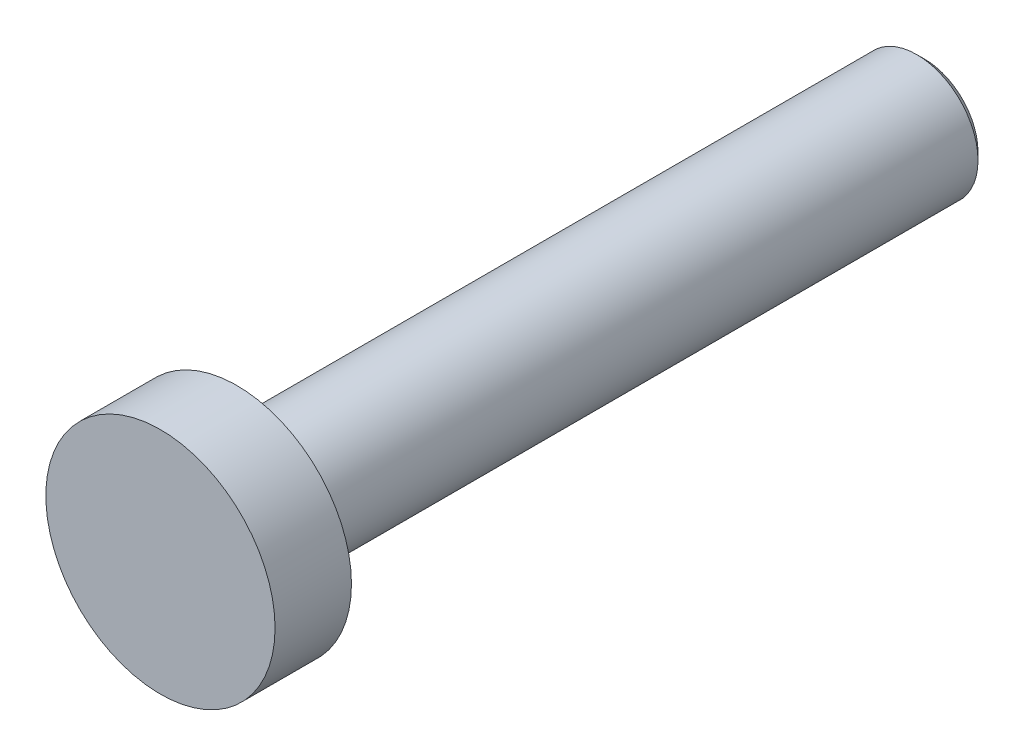
SolidWorks part; units mm, degrees
ref_plane "Front Plane" through (0, 0, 0) normal (0, 0, 1) x (1, 0, 0)
ref_plane "Top Plane" through (0, 0, 0) normal (0, 1, 0) x (1, 0, 0)
ref_plane "Right Plane" through (0, 0, 0) normal (1, 0, 0) x (0, 0, -1)
sketch "Sketch1" plane through (0, 0, 0) normal (0, 0, 1) x (1, 0, 0)
  circle A0 centre (0, 0) radius 4
  dimension "D1" = 8
extrude "Boss-Extrude1" add sketch "Sketch1" along normal blind 45
sketch "Sketch2" plane through (0, 0, 45) normal (0, 0, 1) x (1, 0, 0)
  circle A0 centre (0, 0) radius 7.5
  dimension "D1" = 15
extrude "Boss-Extrude2" add sketch "Sketch2" along normal blind 5
chamfer "Chamfer1" distance 0.5 angle 45 1 edges at (4, 0, 0)
